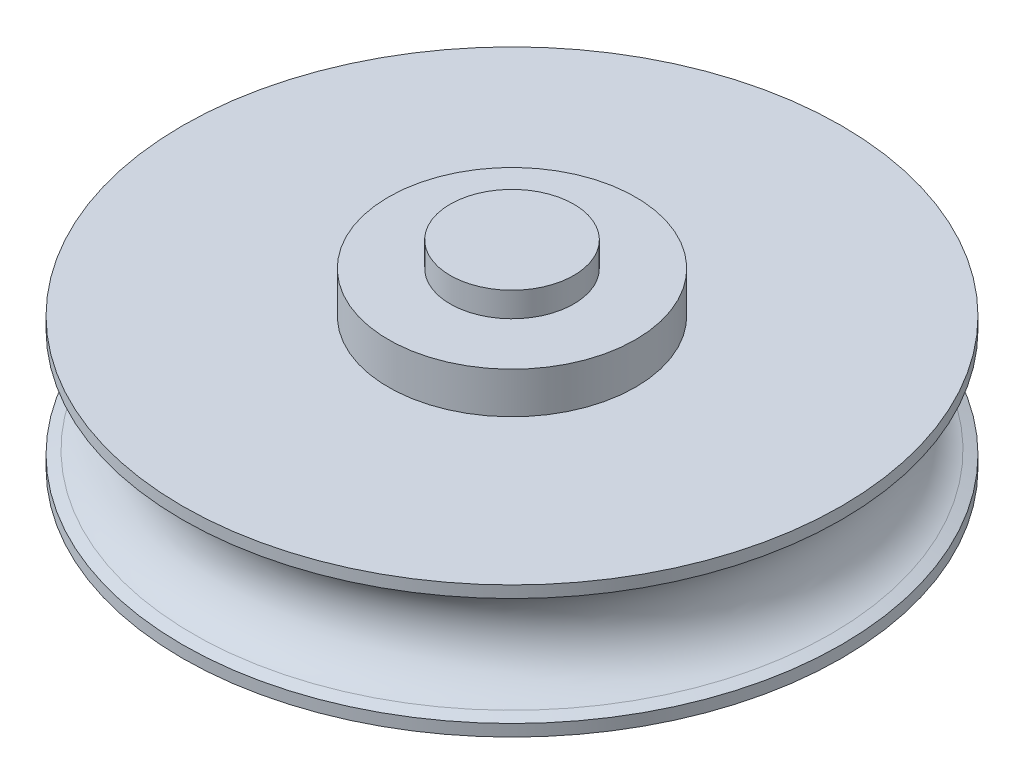
from build123d import *


with BuildPart() as part:
    # Sketch1 → Revolve1 (revolve)
    with BuildSketch(Plane.XY):
        with BuildLine():
            Line((-15, 0), (-40, 0))
            Line((-40, 0), (-40, 1.432640688))
            Line((-40, 1.432640688), (-38.716216216, 1.914416082))
            ThreePointArc((-38.716216216, 1.914416082), (-34.5, 8), (-38.716216216, 14.085583918))
            Line((-38.716216216, 14.085583918), (-40, 14.567359312))
            Line((-40, 14.567359312), (-40, 16))
            Line((-40, 16), (-15, 16))
            Line((-15, 16), (-15, 21))
            Line((-15, 21), (-7.5, 21))
            Line((-7.5, 21), (-7.5, 24))
            Line((-7.5, 24), (0, 24))
            Line((0, 24), (0, -8))
            Line((0, -8), (-7.5, -8))
            Line((-7.5, -8), (-7.5, -5))
            Line((-7.5, -5), (-15, -5))
            Line((-15, -5), (-15, 0))
        make_face()
    revolve(axis=Axis((0, 24, 0), (0, -1, 0)))


solid = part.part
